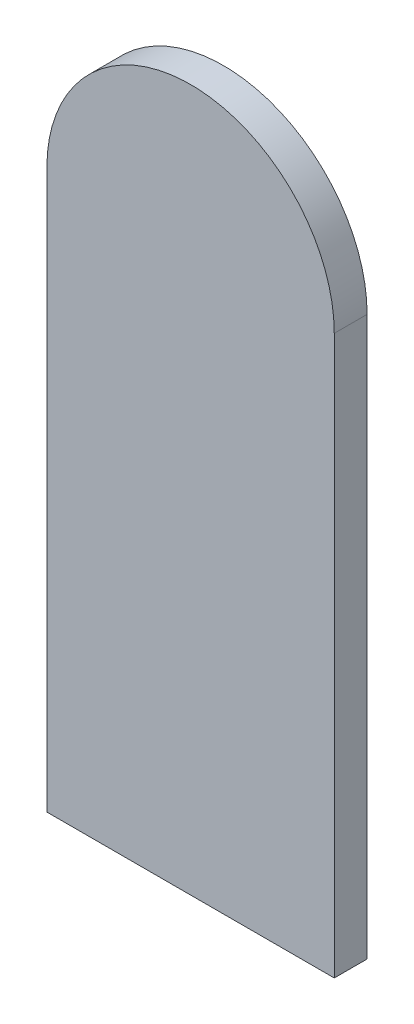
from build123d import *

# Parameters (mm, degrees)
EXTRUDE_1_DEPTH = 4


with BuildPart() as part:
    # 草图1 → 凸台-拉伸1 (new body)
    with BuildSketch(Plane.XY):
        with BuildLine():
            Line((0, 0), (-17.5, 0))
            Line((-17.5, 0), (-17.5, 68))
            ThreePointArc((-17.5, 68), (0, 85.5), (17.5, 68))
            Line((17.5, 68), (17.5, 0))
            Line((17.5, 0), (0, 0))
        make_face()
    extrude(amount=EXTRUDE_1_DEPTH)


solid = part.part
